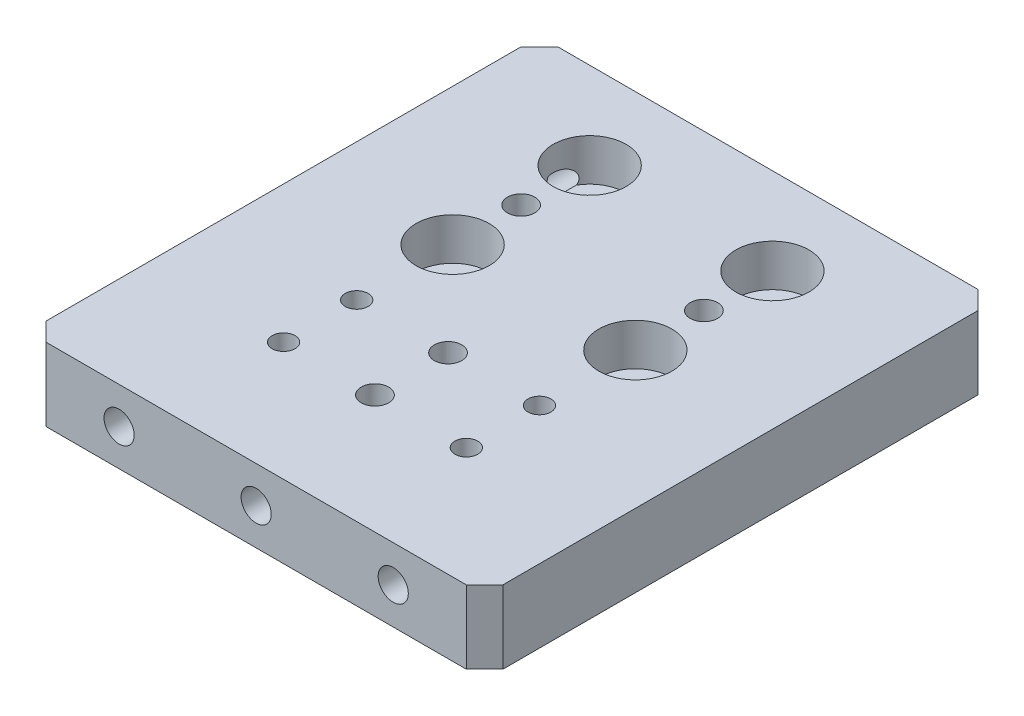
SolidWorks part; units mm, degrees
material "A6061 T6"
ref_plane "前视基准面" through (0, 0, 0) normal (0, 0, 1) x (1, 0, 0)
ref_plane "上视基准面" through (0, 0, 0) normal (0, 1, 0) x (1, 0, 0)
ref_plane "右视基准面" through (0, 0, 0) normal (1, 0, 0) x (0, 0, -1)
sketch "草图1" plane through (0, 0, 0) normal (0, 1, 0) x (1, 0, 0)
  line L1 (-25, 28) -> (25, 28)
  line L2 (-25, 28) -> (-25, -28)
  line L3 (-25, -28) -> (25, -28)
  line L4 (25, 28) -> (25, -28)
  line L5 (-25, 28) -> (25, -28) construction
  line L6 (-25, -28) -> (25, 28) construction
  point P0 (0, 0)
  dimension "D1" = 50
  dimension "D2" = 56
extrude "凸台-拉伸1" add sketch "草图1" along normal blind 8
hole_wizard "M4 螺纹孔1" positions "草图2" profile "草图3" tap size "M4" standard "GB"
sketch "草图2" plane through (0, 0, 28) normal (0, 0, 1) x (1, 0, 0)
  line L0 (25, 8) -> (25, 0) construction
  line L1 (-25, 8) -> (-25, 0) construction
  line L2 (-25, 0) -> (25, 0) construction
  point P0 (15, 4)
  point P2 (0, 4)
  point P4 (-15, 4)
  dimension "D1" = 10
  dimension "D2" = 10
  dimension "D3" = 15
  dimension "D4" = 4
sketch "草图3" plane through (15, 4, 28) normal (1, 0, 0) x (0, -1, 0)
  line L0 (0, 0) -> (0, 11.0914)
  line L1 (0, 11.0914) -> (1.65, 10.1)
  line L2 (1.65, 10.1) -> (1.65, 0)
  line L5 (1.65, 0) -> (0, 0)
  line L10 (0, 11.0914) -> (-1.65, 10.1) construction
  line L11 (0, -6.35) -> (0, 107.95) construction
  dimension "螺纹孔钻头直径" = 3.3
  dimension "螺纹孔钻头深度" = 10.1
  dimension "导头角度" = 118
cosmetic thread "孔螺蚊线1"
cosmetic thread "孔螺蚊线2"
cosmetic thread "孔螺蚊线3"
chamfer "倒角1" distance 2 angle 45 2 edges at (-25, 4, 28) (25, 4, 28)
hole_wizard "M4 螺纹孔2" positions "草图4" profile "草图5" tap size "M4" standard "GB"
sketch "草图4" plane through (0, 0, -28) normal (0, 0, -1) x (-1, 0, 0)
  line L0 (-25, 8) -> (25, 8) construction
  line L3 (-25, 8) -> (-25, 0) construction
  line L4 (25, 8) -> (25, 0) construction
  point P0 (-15, 4)
  point P2 (0, 4)
  point P4 (15, 4)
  dimension "D1" = 4
  dimension "D2" = 10
  dimension "D3" = 10
  dimension "D4" = 15
sketch "草图5" plane through (15, 4, -28) normal (1, 0, 0) x (0, 1, 0)
  line L0 (0, 0) -> (0, 11.0914)
  line L1 (0, 11.0914) -> (1.65, 10.1)
  line L2 (1.65, 10.1) -> (1.65, 0)
  line L5 (1.65, 0) -> (0, 0)
  line L10 (0, 11.0914) -> (-1.65, 10.1) construction
  line L11 (0, -6.35) -> (0, 107.95) construction
  dimension "螺纹孔钻头直径" = 3.3
  dimension "螺纹孔钻头深度" = 10.1
  dimension "导头角度" = 118
cosmetic thread "孔螺蚊线4"
cosmetic thread "孔螺蚊线5"
cosmetic thread "孔螺蚊线6"
hole_wizard "大小mm 暗销孔1" positions "草图6" profile "草图7" hole size "Ø3.0" standard "GB"
sketch "草图6" plane through (0, 0, 0) normal (0, -1, 0) x (-1, 0, 0)
  point P0 (0, -7)
  point P3 (0, -15)
sketch "草图7" plane through (0, 0, 7) normal (1, 0, 0) x (0, 0, -1)
  line L0 (0, 0) -> (0, 13.3013)
  line L1 (0, 13.3013) -> (1.5, 12.4)
  line L2 (1.5, 12.4) -> (1.5, 0)
  line L5 (1.5, 0) -> (0, 0)
  line L10 (0, 13.3013) -> (-1.5, 12.4) construction
  line L11 (0, -6.35) -> (0, 107.95) construction
  dimension "孔直径" = 3
  dimension "孔深度" = 12.4
  dimension "导头角度" = 118
hole_wizard "M3 螺纹孔1" positions "草图8" profile "草图9" tap size "M3" standard "GB"
sketch "草图8" plane through (0, 0, 0) normal (0, -1, 0) x (-1, 0, 0)
  point P0 (-10, -7)
  point P3 (10, -7)
  point P6 (-10, -15)
  point P9 (10, -15)
sketch "草图9" plane through (10, 0, 7) normal (1, 0, 0) x (0, 0, -1)
  line L0 (0, 0) -> (0, 15.7511)
  line L1 (0, 15.7511) -> (1.25, 15)
  line L2 (1.25, 15) -> (1.25, 0)
  line L5 (1.25, 0) -> (0, 0)
  line L10 (0, 15.7511) -> (-1.25, 15) construction
  line L11 (0, -6.35) -> (0, 107.95) construction
  dimension "螺纹孔钻头直径" = 2.5
  dimension "螺纹孔钻头深度" = 15
  dimension "导头角度" = 118
cosmetic thread "孔螺蚊线7"
cosmetic thread "孔螺蚊线8"
cosmetic thread "孔螺蚊线9"
cosmetic thread "孔螺蚊线10"
hole_wizard "大小mm 暗销孔2" positions "草图14" profile "草图13" hole size "Ø3.0" standard "GB"
sketch "草图14" plane through (0, 8, 0) normal (0, 1, 0) x (1, 0, 0)
  point P0 (-10, 11)
sketch "草图13" plane through (-10, 8, -11) normal (1, 0, 0) x (0, 0, 1)
  line L0 (0, 0) -> (0, 15.9013)
  line L1 (0, 15.9013) -> (1.5, 15)
  line L2 (1.5, 15) -> (1.5, 0)
  line L5 (1.5, 0) -> (0, 0)
  line L10 (0, 15.9013) -> (-1.5, 15) construction
  line L11 (0, -6.35) -> (0, 107.95) construction
  dimension "孔直径" = 3
  dimension "孔深度" = 15
  dimension "导头角度" = 118
hole_wizard "打孔尺寸(%根据)内六角圆柱头螺钉的类型1" positions "草图15" profile "草图16" counterbore size "M4" standard "GB"
sketch "草图15" plane through (0, 8, 0) normal (0, 1, 0) x (1, 0, 0)
  point P0 (-10, 18.5)
  point P3 (-10, 3.5)
sketch "草图16" plane through (-10, 8, -18.5) normal (1, 0, 0) x (0, 0, 1)
  line L0 (0, 0) -> (0, 16.3519)
  line L1 (0, 16.3519) -> (2.25, 15)
  line L2 (2.25, 15) -> (2.25, 4.6)
  line L3 (2.25, 4.6) -> (4, 4.6)
  line L4 (4, 4.6) -> (4, 0)
  line L5 (4, 0) -> (0, 0)
  line L10 (0, 16.3519) -> (-2.25, 15) construction
  line L11 (0, -6.35) -> (0, 107.95) construction
  dimension "孔直径" = 4.5
  dimension "孔深度" = 15
  dimension "柱形沉头孔直径" = 8
  dimension "柱形沉头孔深度" = 4.6
  dimension "导头角度" = 118
hole_wizard "打孔尺寸(%根据)内六角圆柱头螺钉的类型2" positions "草图17" profile "草图18" counterbore size "M4" standard "GB"
sketch "草图17" plane through (0, 8, 0) normal (0, 1, 0) x (1, 0, 0)
  point P0 (10, 18.5)
  point P3 (10, 3.5)
sketch "草图18" plane through (10, 8, -18.5) normal (1, 0, 0) x (0, 0, 1)
  line L0 (0, 0) -> (0, 16.3519)
  line L1 (0, 16.3519) -> (2.25, 15)
  line L2 (2.25, 15) -> (2.25, 4.6)
  line L3 (2.25, 4.6) -> (4, 4.6)
  line L4 (4, 4.6) -> (4, 0)
  line L5 (4, 0) -> (0, 0)
  line L10 (0, 16.3519) -> (-2.25, 15) construction
  line L11 (0, -6.35) -> (0, 107.95) construction
  dimension "孔直径" = 4.5
  dimension "孔深度" = 15
  dimension "柱形沉头孔直径" = 8
  dimension "柱形沉头孔深度" = 4.6
  dimension "导头角度" = 118
hole_wizard "大小mm 暗销孔3" positions "草图19" profile "草图20" hole size "Ø3.0" standard "GB"
sketch "草图19" plane through (0, 8, 0) normal (0, 1, 0) x (1, 0, 0)
  point P0 (10, 11)
sketch "草图20" plane through (10, 8, -11) normal (1, 0, 0) x (0, 0, 1)
  line L0 (0, 0) -> (0, 15.9013)
  line L1 (0, 15.9013) -> (1.5, 15)
  line L2 (1.5, 15) -> (1.5, 0)
  line L5 (1.5, 0) -> (0, 0)
  line L10 (0, 15.9013) -> (-1.5, 15) construction
  line L11 (0, -6.35) -> (0, 107.95) construction
  dimension "孔直径" = 3
  dimension "孔深度" = 15
  dimension "导头角度" = 118
chamfer "倒角2" distance 2 angle 45 2 edges at (25, 4, -28) (-25, 4, -28)
